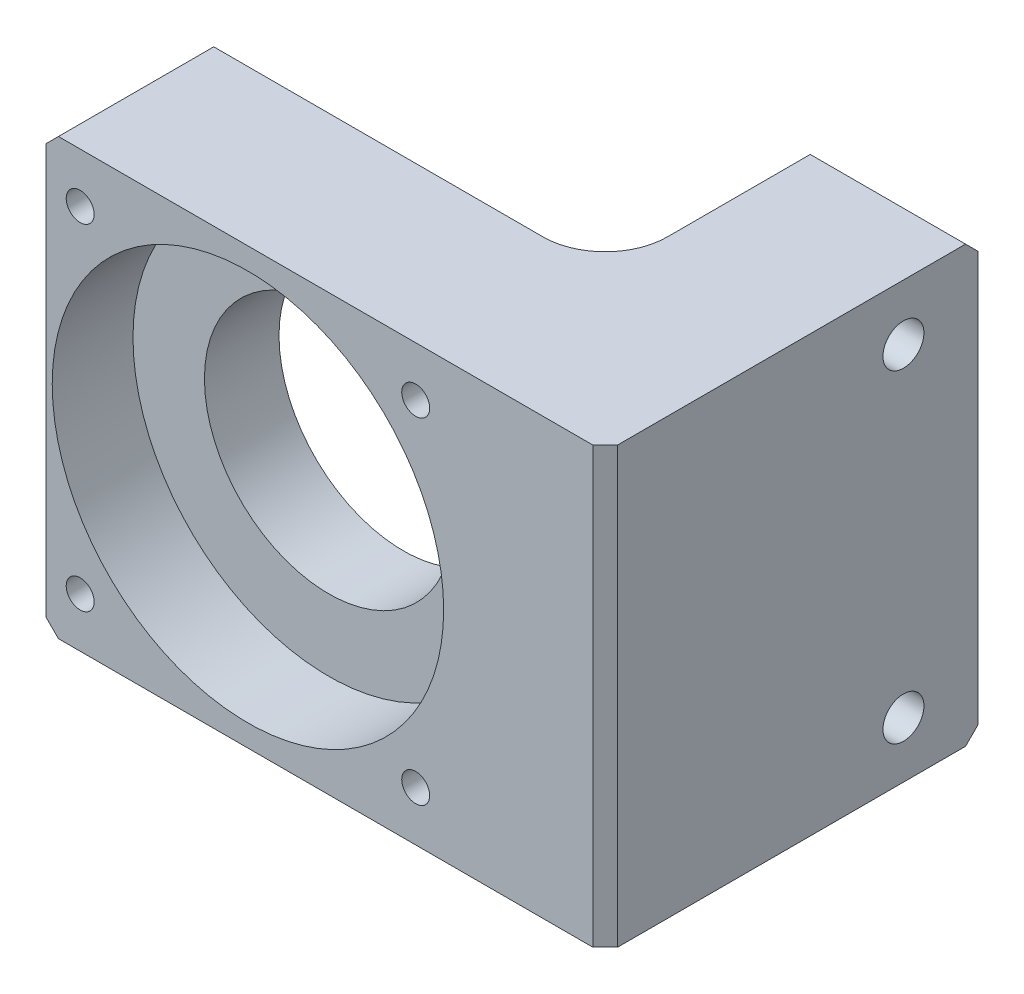
SolidWorks part; units mm, degrees
ref_plane "前视基准面" through (0, 0, 0) normal (0, 0, 1) x (1, 0, 0)
ref_plane "上视基准面" through (0, 0, 0) normal (0, 1, 0) x (1, 0, 0)
ref_plane "右视基准面" through (0, 0, 0) normal (1, 0, 0) x (0, 0, -1)
sketch "草图1" plane through (0, 0, 0) normal (0, 1, 0) x (1, 0, 0)
  line L0 (0, 0) -> (90, 0)
  line L1 (90, 0) -> (90, 60)
  line L2 (90, 60) -> (65, 60)
  line L3 (65, 60) -> (65, 25)
  line L4 (65, 25) -> (0, 25)
  line L5 (0, 25) -> (0, 0)
  dimension "D1" = 25
  dimension "D2" = 25
  dimension "D3" = 90
  dimension "D4" = 60
extrude "凸台-拉伸1" add sketch "草图1" along normal mid plane 70
fillet "圆角1" radius 10 1 edges at (65, 0, -25)
sketch "草图2" plane through (0, 0, 0) normal (0, 0, 1) x (1, 0, 0)
  circle A0 centre (32.5, 0) radius 31.5
  dimension "D1" = 63
  dimension "D2" = 32.5
extrude "切除-拉伸1" cut sketch "草图2" against normal blind 13
sketch "草图3" plane through (0, 0, -25) normal (0, 0, -1) x (-1, 0, 0)
  circle A0 centre (-32.5, 0) radius 20
  dimension "D1" = 40
  dimension "D2" = 32.5
extrude "切除-拉伸2" cut sketch "草图3" against normal through all both and the other way through all
sketch "草图6" plane through (65, 0, 0) normal (-1, 0, 0) x (0, 0, 1)
  line L0 (0, 0) -> (-72.7297, 0) construction
  line L2 (-60, 35) -> (-60, -35) construction
  point P0 (-48, 26)
  point P2 (-48, -26)
  dimension "D1" = 52
  dimension "D2" = 12
hole_wizard "M6 六角圆柱头螺钉的柱形沉头孔1" positions "草图6" profile "草图5" counterbore size "M6" standard "GB" end condition through all
sketch "草图5" plane through (65, 26, -48) normal (0, 1, 0) x (0, 0, 1)
  line L0 (0, 0) -> (0, 25)
  line L1 (0, 25) -> (3.3, 25)
  line L3 (3.3, 25) -> (3.3, 6.8)
  line L4 (3.3, 6.8) -> (5.5, 6.8)
  line L5 (5.5, 6.8) -> (5.5, 0)
  line L7 (5.5, 0) -> (0, 0)
  line L11 (0, -6.35) -> (0, 107.95) construction
  dimension "通孔孔直径" = 6.6
  dimension "通孔孔深度" = 25
  dimension "柱形沉头孔直径" = 11
  dimension "柱形沉头孔深度" = 6.8
chamfer "倒角1" distance 2 angle 45 5 edges at (90, 0, 0) (77.5, 35, -60) (77.5, -35, -60) (0, 35, -12.5) (0, -35, -12.5)
sketch "草图9" plane through (0, 0, -60) normal (0, 0, -1) x (-1, 0, 0)
  point P0 (-5.5, 27)
  point P3 (-59.5, 27)
  point P6 (-59.5, -27)
  point P9 (-5.5, -27)
hole_wizard "M4 六角圆柱头螺钉的柱形沉头孔1" positions "草图9" profile "草图8" counterbore size "M4" standard "GB" end condition through all
sketch "草图8" plane through (5.5, 27, -60) normal (1, 0, 0) x (0, 1, 0)
  line L0 (0, 0) -> (0, 60)
  line L1 (0, 60) -> (2.25, 60)
  line L3 (2.25, 60) -> (2.25, 43.6)
  line L4 (2.25, 43.6) -> (4, 43.6)
  line L5 (4, 43.6) -> (4, 0)
  line L7 (4, 0) -> (0, 0)
  line L11 (0, -6.35) -> (0, 107.95) construction
  dimension "通孔孔直径" = 4.5
  dimension "通孔孔深度" = 60
  dimension "柱形沉头孔直径" = 8
  dimension "柱形沉头孔深度" = 43.6
